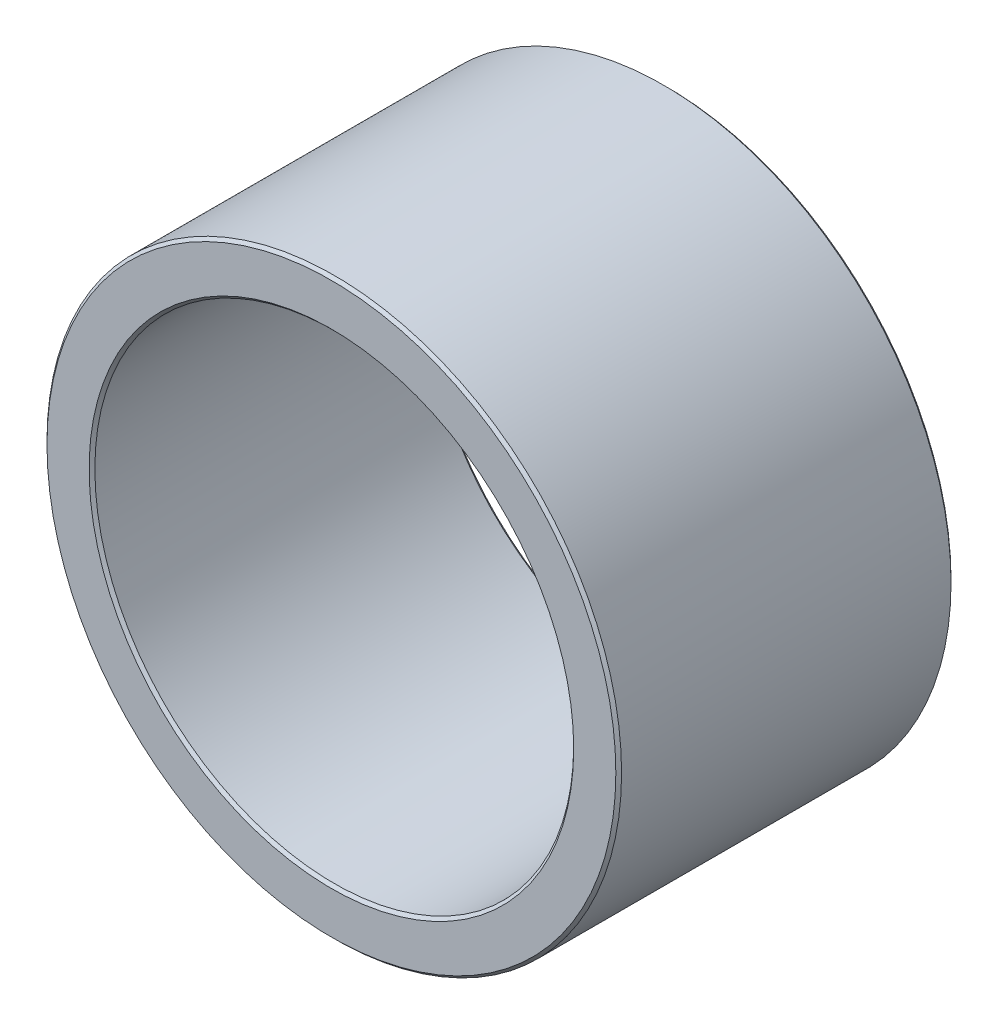
SolidWorks part; units mm, degrees
material "铝青铜"
ref_plane "Front Plane" through (0, 0, 0) normal (0, 0, 1) x (1, 0, 0)
ref_plane "Top Plane" through (0, 0, 0) normal (0, 1, 0) x (1, 0, 0)
ref_plane "Right Plane" through (0, 0, 0) normal (1, 0, 0) x (0, 0, -1)
sketch "Sketch1" plane through (0, 0, 0) normal (0, 0, 1) x (1, 0, 0)
  circle A0 centre (0, 0) radius 30
  circle A1 centre (0, 0) radius 25
  dimension "D1" = 50
  dimension "D2" = 60
extrude "Boss-Extrude1" add sketch "Sketch1" along normal blind 35
chamfer "Chamfer1" distance 0.3 angle 45 4 edges at (30, 0, 0) (30, 0, 35) (25, 0, 0) (25, 0, 35)
